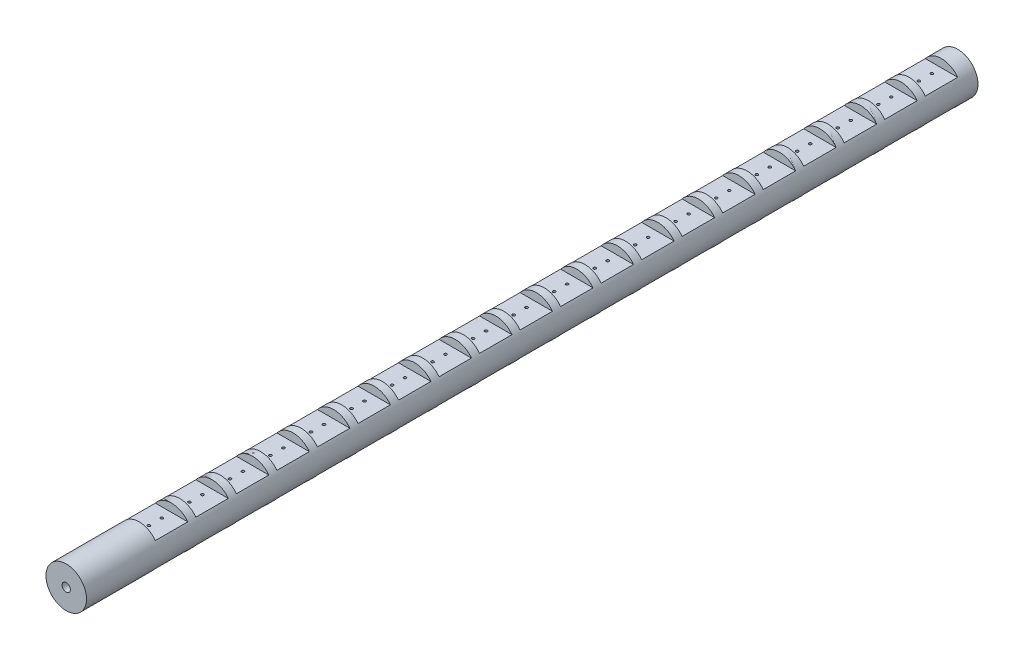
SolidWorks part; units mm, degrees
ref_plane "Front Plane" through (0, 0, 0) normal (0, 0, 1) x (1, 0, 0)
ref_plane "Top Plane" through (0, 0, 0) normal (0, 1, 0) x (1, 0, 0)
ref_plane "Right Plane" through (0, 0, 0) normal (1, 0, 0) x (0, 0, -1)
sketch "Sketch1" plane through (0, 0, 0) normal (0, 0, 1) x (1, 0, 0)
  circle A0 centre (0, 0) radius 25
  dimension "D1" = 50
extrude "Boss-Extrude1" add sketch "Sketch1" along normal blind 1100
hole_wizard "M12 Tapped Hole1" positions "3DSketch2" profile "Sketch2" tap size "M12" standard "GB"
sketch3d "3DSketch2"
  circle A0 centre (0, 0, 1100) radius 25 construction
  point P0 (0, 0, 1100)
  point P6 (0, 0, 1125)
sketch "Sketch2" plane through (0, 0, 1100) normal (1, 0, 0) x (0, -1, 0)
  line L0 (0, 0) -> (0, 32.3144)
  line L1 (0, 32.3144) -> (5.1, 29.25)
  line L2 (5.1, 29.25) -> (5.1, 0)
  line L5 (5.1, 0) -> (0, 0)
  line L10 (0, 32.3144) -> (-5.1, 29.25) construction
  line L11 (0, -6.35) -> (0, 107.95) construction
  dimension "螺纹孔钻头直径" = 10.2
  dimension "螺纹孔钻头深度" = 29.25
  dimension "导头角度" = 118
cosmetic thread "Cosmetic Thread 1" parameters "D1"=24, "D2"=12
sketch "Sketch3" plane through (0, 0, 0) normal (0, 0, -1) x (-1, 0, 0)
  circle A0 centre (0, 0) radius 10
  dimension "D1" = 20
extrude "Cut-Extrude1" cut sketch "Sketch3" against normal blind 484
sketch "Sketch4" plane through (0, 0, 0) normal (0, 1, 0) x (1, 0, 0)
  line L1 (-25, -20) -> (25, -20)
  line L2 (-25, -20) -> (-25, -60)
  line L3 (-25, -60) -> (25, -60)
  line L4 (25, -20) -> (25, -60)
  line L5 (-25, -20) -> (25, -60) construction
  line L6 (-25, -60) -> (25, -20) construction
  point P0 (0, -40)
  dimension "D1" = 40
  dimension "D2" = 50
  dimension "D3" = 20
extrude "Cut-Extrude2" cut sketch "Sketch4" against normal blind 484 from offset 15 offset against normal yes
sketch "Sketch5" plane through (0, -15, 0) normal (0, -1, 0) x (1, 0, 0)
  line L0 (0, 60) -> (0, 20) construction
  line L1 (-20, 60) -> (20, 60) construction
  line L2 (20, 20) -> (-20, 20) construction
  line L3 (-20, 60) -> (20, 60) construction
  line L4 (20, 20) -> (-20, 20) construction
  point P6 (0, 48)
  point P7 (0, 32)
  dimension "D1" = 12
  dimension "D2" = 12
hole_wizard "M4 Tapped Hole1" positions "3DSketch3" profile "Sketch6" tap size "M4" standard "GB"
sketch3d "3DSketch3"
  point P0 (0, -15, 48)
  point P3 (0, -15, 32)
sketch "Sketch6" plane through (0, -15, 48) normal (1, 0, 0) x (0, 0, -1)
  line L0 (0, 0) -> (0, 11.0914)
  line L1 (0, 11.0914) -> (1.65, 10.1)
  line L2 (1.65, 10.1) -> (1.65, 0)
  line L5 (1.65, 0) -> (0, 0)
  line L10 (0, 11.0914) -> (-1.65, 10.1) construction
  line L11 (0, -6.35) -> (0, 107.95) construction
  dimension "螺纹孔钻头直径" = 3.3
  dimension "螺纹孔钻头深度" = 10.1
  dimension "导头角度" = 118
cosmetic thread "Cosmetic Thread 2" parameters "D1"=5.1371, "D2"=4
cosmetic thread "Cosmetic Thread 3" parameters "D1"=5.1371, "D2"=4
pattern_linear "LPattern1" count 20 spacing 50 along (0, 0, 1) of "Cut-Extrude2", "M4 Tapped Hole1"
mirror "Mirror1" about plane through (0, 0, 0) normal (0, 1, 0) of "LPattern1", "Cut-Extrude2", "M4 Tapped Hole1"
hole_wizard "M4 Tapped Hole2" positions "3DSketch4" profile "Sketch8" tap size "M4" standard "GB"
sketch3d "3DSketch4"
  point P0 (16.8594, 0.5135, 0)
  point P2 (-17.7152, -0.1712, 0)
sketch "Sketch8" plane through (16.8594, 0.5135, 0) normal (1, 0, 0) x (0, 1, 0)
  line L0 (0, 0) -> (0, 11.0914)
  line L1 (0, 11.0914) -> (1.65, 10.1)
  line L2 (1.65, 10.1) -> (1.65, 0)
  line L5 (1.65, 0) -> (0, 0)
  line L10 (0, 11.0914) -> (-1.65, 10.1) construction
  line L11 (0, -6.35) -> (0, 107.95) construction
  dimension "螺纹孔钻头直径" = 3.3
  dimension "螺纹孔钻头深度" = 10.1
  dimension "导头角度" = 118
cosmetic thread "Cosmetic Thread 4" parameters "D1"=8, "D2"=4
cosmetic thread "Cosmetic Thread 5" parameters "D1"=8, "D2"=4
